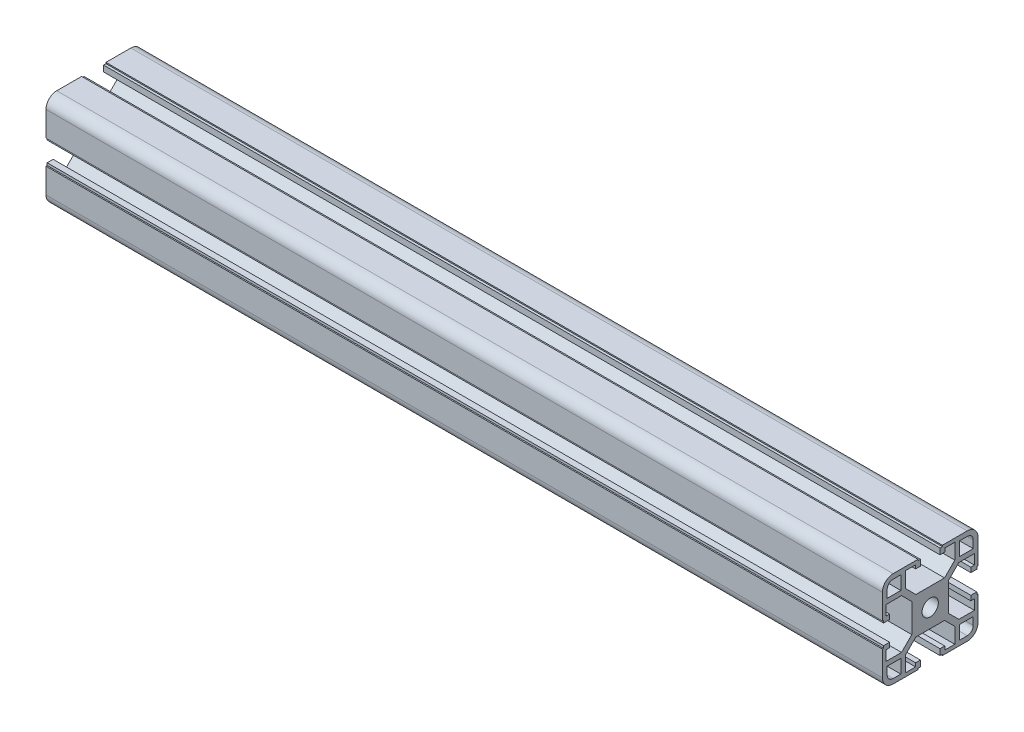
SolidWorks part; units mm, degrees
ref_plane "Front Plane" through (0, 0, 0) normal (0, 0, 1) x (1, 0, 0)
ref_plane "Top Plane" through (0, 0, 0) normal (0, 1, 0) x (1, 0, 0)
ref_plane "Right Plane" through (0, 0, 0) normal (1, 0, 0) x (0, 0, -1)
sketch "草图1" plane through (0, 0, 0) normal (0, 0, 1) x (1, 0, 0)
  line L0 (-984.975, 0) -> (-634.975, 0)
  dimension "D1" = 350
other "Aluminium profile 40 X 40B X R4.5(1)"
ref_plane "Plane1" through (-984.975, 0, 0) normal (1, 0, 0) x (0, 1, 0)
sketch "Sketch1" plane through (-984.975, 0, 0) normal (1, 0, 0) x (0, 1, 0)
  line L0 (-5.1, 20) -> (-5.1, 19.5)
  line L1 (-5.1, 19.5) -> (-4.1, 19.5)
  line L2 (-4.1, 19.5) -> (-4.1, 17)
  line L3 (-6.1, 18.5) -> (-10.3, 18.5)
  line L4 (-15.5, -20) -> (-5.1, -20)
  line L5 (-20, -15.5) -> (-20, -5.1)
  line L6 (15.5, 20) -> (5.1, 20)
  line L7 (20, 15.5) -> (20, 5.1)
  line L8 (0, 14.8756) -> (0, 0) construction
  line L9 (0, 0) -> (14.1675, 0) construction
  line L10 (-10.3, 18.5) -> (-10.3, 12)
  line L11 (-10.3, 12) -> (-6, 7.7)
  line L12 (-6, 7.7) -> (6, 7.7)
  line L13 (10.3, 12) -> (6, 7.7)
  line L14 (10.3, 18.5) -> (10.3, 12)
  line L15 (6.1, 18.5) -> (10.3, 18.5)
  line L16 (4.1, 19.5) -> (4.1, 17)
  line L17 (5.1, 19.5) -> (4.1, 19.5)
  line L18 (5.1, 20) -> (5.1, 19.5)
  line L19 (-5.1, 20) -> (-15.5, 20)
  line L20 (20, 5.1) -> (19.5, 5.1)
  line L21 (12.3, 18) -> (15.5, 18)
  line L22 (12.3, 18) -> (12.3, 12.3)
  line L23 (12.3, 12.3) -> (18, 12.3)
  line L24 (18, 15.5) -> (18, 12.3)
  line L25 (19.5, 5.1) -> (19.5, 4.1)
  line L26 (19.5, 4.1) -> (17, 4.1)
  line L27 (17, 6.1) -> (17, 4.1)
  line L28 (18.5, 6.1) -> (17, 6.1)
  line L29 (18.5, 6.1) -> (18.5, 10.3)
  line L30 (18.5, 10.3) -> (12, 10.3)
  line L31 (12, 10.3) -> (7.7, 6)
  line L32 (7.7, 6) -> (7.7, -6)
  line L33 (12, -10.3) -> (7.7, -6)
  line L34 (18.5, -10.3) -> (12, -10.3)
  line L35 (18.5, -6.1) -> (18.5, -10.3)
  line L36 (18.5, -6.1) -> (17, -6.1)
  line L37 (17, -4.1) -> (17, -6.1)
  line L38 (19.5, -4.1) -> (17, -4.1)
  line L39 (19.5, -5.1) -> (19.5, -4.1)
  line L40 (20, -5.1) -> (19.5, -5.1)
  line L41 (5.1, -20) -> (5.1, -19.5)
  line L42 (5.1, -19.5) -> (4.1, -19.5)
  line L43 (4.1, -19.5) -> (4.1, -17)
  line L44 (6.1, -17) -> (4.1, -17)
  line L45 (6.1, -18.5) -> (6.1, -17)
  line L46 (6.1, -18.5) -> (10.3, -18.5)
  line L47 (10.3, -18.5) -> (10.3, -12)
  line L48 (10.3, -12) -> (6, -7.7)
  line L49 (6, -7.7) -> (-6, -7.7)
  line L50 (-10.3, -12) -> (-6, -7.7)
  line L51 (-10.3, -18.5) -> (-10.3, -12)
  line L52 (-6.1, -18.5) -> (-10.3, -18.5)
  line L53 (-6.1, -18.5) -> (-6.1, -17)
  line L54 (-4.1, -17) -> (-6.1, -17)
  line L55 (-4.1, -19.5) -> (-4.1, -17)
  line L56 (-5.1, -19.5) -> (-4.1, -19.5)
  line L57 (-5.1, -20) -> (-5.1, -19.5)
  line L58 (-20, -5.1) -> (-19.5, -5.1)
  line L59 (5.1, -20) -> (15.5, -20)
  line L60 (-20, 5.1) -> (-20, 15.5)
  line L61 (-19.5, -5.1) -> (-19.5, -4.1)
  line L62 (-6.1, 18.5) -> (-6.1, 17)
  line L63 (-6.1, 17) -> (-4.1, 17)
  line L64 (6.1, 18.5) -> (6.1, 17)
  line L65 (4.1, 17) -> (6.1, 17)
  line L66 (-19.5, -4.1) -> (-17, -4.1)
  line L67 (-15.5, 18) -> (-12.3, 18)
  line L68 (-18, 15.5) -> (-18, 12.3)
  line L69 (-18, 12.3) -> (-12.3, 12.3)
  line L70 (-12.3, 18) -> (-12.3, 12.3)
  line L71 (-17, -6.1) -> (-17, -4.1)
  line L72 (-18.5, -6.1) -> (-17, -6.1)
  line L73 (-18.5, -6.1) -> (-18.5, -10.3)
  line L74 (-18.5, -10.3) -> (-12, -10.3)
  line L75 (-12, -10.3) -> (-7.7, -6)
  line L76 (-7.7, -6) -> (-7.7, 6)
  line L77 (-12, 10.3) -> (-7.7, 6)
  line L78 (-18.5, 10.3) -> (-12, 10.3)
  line L79 (-18.5, 6.1) -> (-18.5, 10.3)
  line L80 (-18.5, 6.1) -> (-17, 6.1)
  line L81 (-17, 4.1) -> (-17, 6.1)
  line L82 (-19.5, 4.1) -> (-17, 4.1)
  line L83 (-19.5, 5.1) -> (-19.5, 4.1)
  line L84 (-20, 5.1) -> (-19.5, 5.1)
  line L85 (20, -5.1) -> (20, -15.5)
  line L87 (-18, -12.3) -> (-12.3, -12.3)
  line L88 (-18, -12.3) -> (-18, -15.5)
  line L89 (-15.5, -18) -> (-12.3, -18)
  line L90 (-12.3, -12.3) -> (-12.3, -18)
  line L91 (12.3, -12.3) -> (18, -12.3)
  line L92 (12.3, -12.3) -> (12.3, -18)
  line L93 (12.3, -18) -> (15.5, -18)
  line L94 (18, -12.3) -> (18, -15.5)
  circle A0 centre (0, 0) radius 3.4
  arc A1 (-20, 15.5) -> (-15.5, 20) centre (-15.5, 15.5) cw
  arc A2 (20, 15.5) -> (15.5, 20) centre (15.5, 15.5) ccw
  arc A3 (-15.5, -20) -> (-20, -15.5) centre (-15.5, -15.5) cw
  arc A4 (15.5, -20) -> (20, -15.5) centre (15.5, -15.5) ccw
  arc A5 (-15.5, 18) -> (-18, 15.5) centre (-15.5, 15.5) ccw
  arc A6 (18, 15.5) -> (15.5, 18) centre (15.5, 15.5) ccw
  arc A7 (18, -15.5) -> (15.5, -18) centre (15.5, -15.5) cw
  arc A8 (-18, -15.5) -> (-15.5, -18) centre (-15.5, -15.5) ccw
  point P2 (0, 10)
  point P4 (0, 0)
  point P5 (-20, -20)
  point P6 (20, -20)
  point P7 (20, 20)
  point P8 (-20, 20)
  point P36 (-20, 20)
  point P39 (20, 20)
  point P121 (0, 0)
  dimension "D1" = 20.6
  dimension "D2" = 40
  dimension "D3" = 8.2
  dimension "D4" = 10.2
  dimension "D5" = 12.3
  dimension "D6" = 6.8
  dimension "D7" = 4.5
  dimension "D8" = 45
  dimension "D12" = 2
  dimension "D13" = 5.7
  dimension "D14" = 2
  dimension "D18" = 2.5
  dimension "D19" = 2.5
  dimension "D15" = 2.5
  dimension "D9" = 0.5
  dimension "D10" = 1.5
  dimension "D11" = 12
  dimension "D16" = 3
  dimension "D17" = 2
  dimension "D20" = 2
  dimension "D21" = 2
